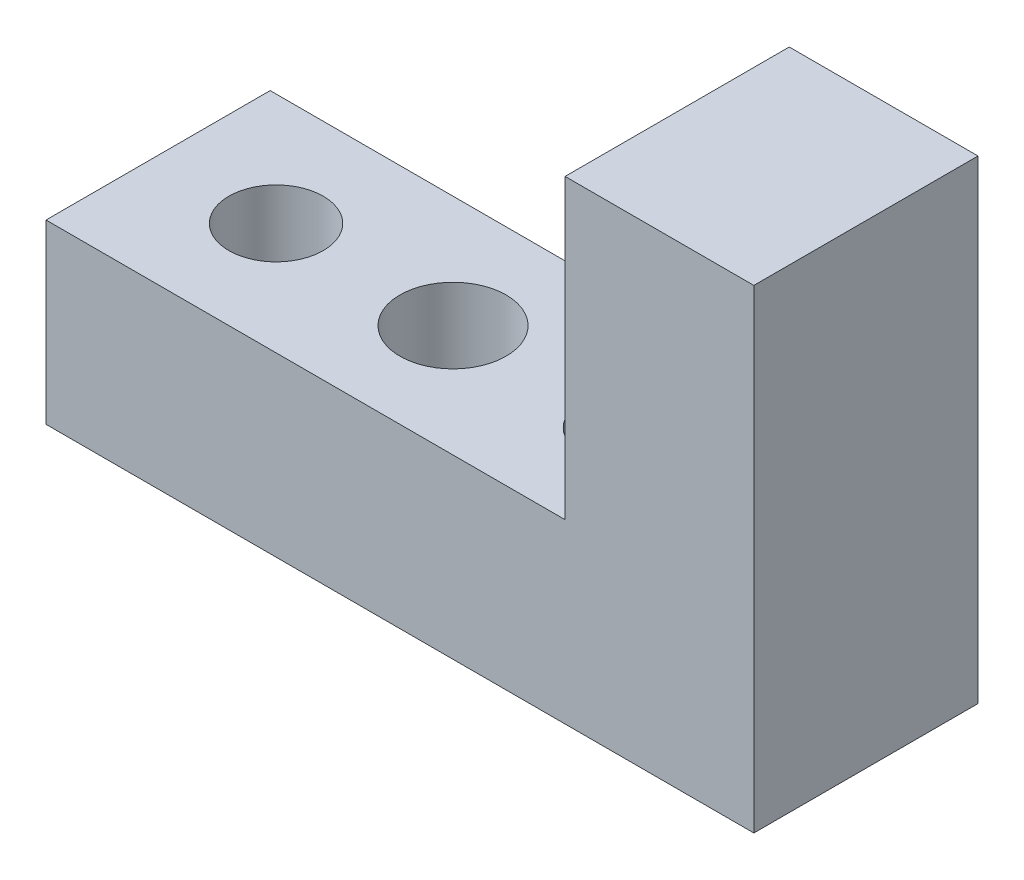
from build123d import *

# Parameters (mm, degrees)
BOSS_EXTRUDE1_DEPTH = 19
SKETCH2_R           = 4
SKETCH2_R_2         = 4.5
CUT_EXTRUDE1_DEPTH  = 15


with BuildPart() as part:
    # Sketch1 → Boss-Extrude1 (new body)
    with BuildSketch(Plane.XY):
        Polygon((0, 0), (60, 0), (60, 40.20000018), (44, 40.20000018), (44, 15), (0, 15), align=None)
    extrude(amount=BOSS_EXTRUDE1_DEPTH)

    # Sketch2 → Cut-Extrude1 (cut)
    with BuildSketch(Plane(origin=(0, 0, 0), x_dir=(-1, 0, 0), z_dir=(0, -1, 0))):
        with Locations(Location((-10, -9.5, 0), (0, 0, 90))):
            Circle(SKETCH2_R)
        with Locations(Location((-25, -9.5, 0), (0, 0, 90))):
            Circle(SKETCH2_R_2)
        with Locations(Location((-40, -9.5, 0), (0, 0, 90))):
            Circle(SKETCH2_R)
    extrude(amount=-CUT_EXTRUDE1_DEPTH, mode=Mode.SUBTRACT)


solid = part.part
